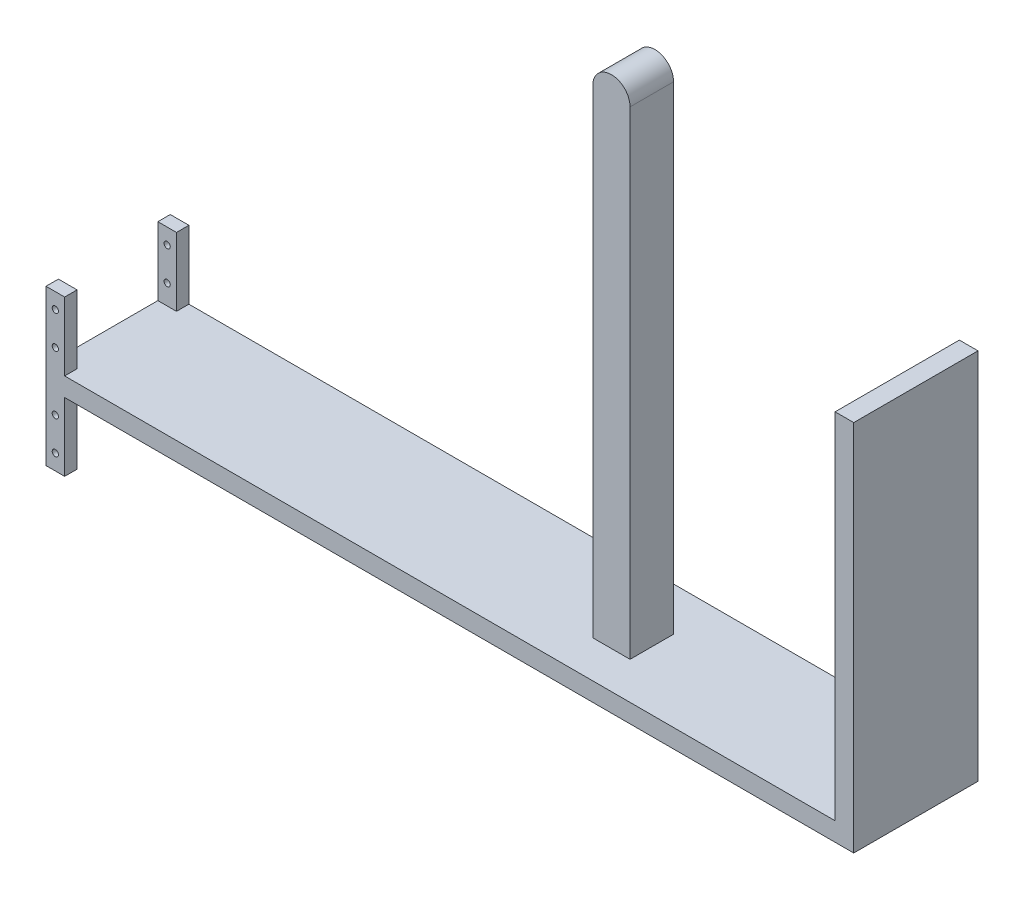
SolidWorks part; units mm, degrees
ref_plane "Front Plane" through (0, 0, 0) normal (0, 0, 1) x (1, 0, 0)
ref_plane "Top Plane" through (0, 0, 0) normal (0, 1, 0) x (1, 0, 0)
ref_plane "Right Plane" through (0, 0, 0) normal (1, 0, 0) x (0, 0, -1)
other "Configuration Table"
sketch "Sketch1" plane through (0, 0, 0) normal (0, 0, 1) x (1, 0, 0)
  line L0 (0, 3.2171) -> (0, -3.2171) construction
  point P4 (0, 0)
sketch "Sketch2" plane through (0, 0, 0) normal (0, 0, 1) x (1, 0, 0)
  line L1 (-148.0502, -835.1984) -> (-178.0502, -835.1984)
  line L2 (-148.0502, -835.1984) -> (-148.0502, -1435.1984)
  line L4 (-178.0502, -835.1984) -> (-178.0502, -1405.1984)
  line L8 (-148.0502, -1435.1984) -> (-1448.0502, -1435.1984)
  line L10 (-178.0502, -1405.1984) -> (-1448.0502, -1405.1984)
  line L11 (-1448.0502, -1435.1984) -> (-1448.0502, -1405.1984)
  dimension "D2" = 30
  dimension "D3" = 1300
  dimension "D4" = 30
extrude "Boss-Extrude1" add sketch "Sketch2" against normal blind 200
sketch "Sketch4" plane through (-1448.0502, 0, 0) normal (-1, 0, 0) x (0, 0, 1)
  line L0 (-100, -1435.1984) -> (-100, -1405.1984) construction
  line L1 (-180, -1295.1984) -> (-200, -1295.1984)
  line L2 (-180, -1295.1984) -> (-180, -1545.1984)
  line L3 (-180, -1545.1984) -> (-200, -1545.1984)
  line L4 (-200, -1295.1984) -> (-200, -1545.1984)
  line L5 (-190, -1545.1984) -> (-190, -1295.1984) construction
  line L6 (-180, -1420.1984) -> (-200, -1420.1984) construction
  line L7 (-200, -1435.1984) -> (0, -1435.1984) construction
  line L8 (-200, -1405.1984) -> (0, -1405.1984) construction
  line L9 (0, -1420.1984) -> (-200, -1420.1984) construction
  line L10 (0, -1405.1984) -> (0, -1435.1984) construction
  line L11 (-200, -1405.1984) -> (-200, -1435.1984) construction
  line L12 (-20, -1420.1984) -> (0, -1420.1984) construction
  line L13 (-10, -1545.1984) -> (-10, -1295.1984) construction
  line L14 (0, -1295.1984) -> (0, -1545.1984)
  line L15 (-20, -1545.1984) -> (0, -1545.1984)
  line L16 (-20, -1295.1984) -> (-20, -1545.1984)
  line L17 (-20, -1295.1984) -> (0, -1295.1984)
  point P0 (-190, -1420.1984)
  point P23 (-10, -1420.1984)
  dimension "D1" = 20
  dimension "D2" = 250
extrude "Boss-Extrude2" add sketch "Sketch4" against normal blind 30
sketch "Sketch5" plane through (0, 0, -200) normal (0, 0, -1) x (-1, 0, 0)
  line L0 (1448.0502, -1420.1984) -> (1418.0502, -1420.1984) construction
  line L1 (1448.0502, -1295.1984) -> (1448.0502, -1545.1984) construction
  line L2 (1433.0502, -1295.1984) -> (1433.0502, -1545.1984) construction
  line L3 (1418.0502, -1295.1984) -> (1448.0502, -1295.1984) construction
  line L4 (1418.0502, -1545.1984) -> (1448.0502, -1545.1984) construction
  line L5 (178.0502, -1405.1984) -> (1418.0502, -1405.1984) construction
  circle A0 centre (1433.0502, -1320.1984) radius 5
  circle A1 centre (1433.0502, -1373.1984) radius 5
  circle A2 centre (1433.0502, -1520.1984) radius 5
  circle A3 centre (1433.0502, -1467.1984) radius 5
  dimension "D1" = 10
  dimension "D2" = 10
  dimension "D3" = 25
  dimension "D4" = 32
extrude "Cut-Extrude1" cut sketch "Sketch5" against normal blind 230
sketch "Sketch9" plane through (0, 0, 0) normal (0, 0, 1) x (1, 0, 0)
  line L0 (-178.0502, -1405.1984) -> (-1418.0502, -1405.1984) construction
  line L1 (-568.0502, -1405.1984) -> (-628.0502, -1405.1984)
  line L2 (-568.0502, -1405.1984) -> (-568.0502, -635.1984)
  line L4 (-628.0502, -1405.1984) -> (-628.0502, -635.1984)
  line L5 (-178.0502, -835.1984) -> (-178.0502, -1405.1984) construction
  arc A0 (-568.0502, -635.1984) -> (-628.0502, -635.1984) centre (-598.0502, -635.1984) ccw
  dimension "D3" = 800
  dimension "D1" = 390
  dimension "D2" = 60
extrude "Boss-Extrude5" add sketch "Sketch9" against normal blind 70 from offset 60
